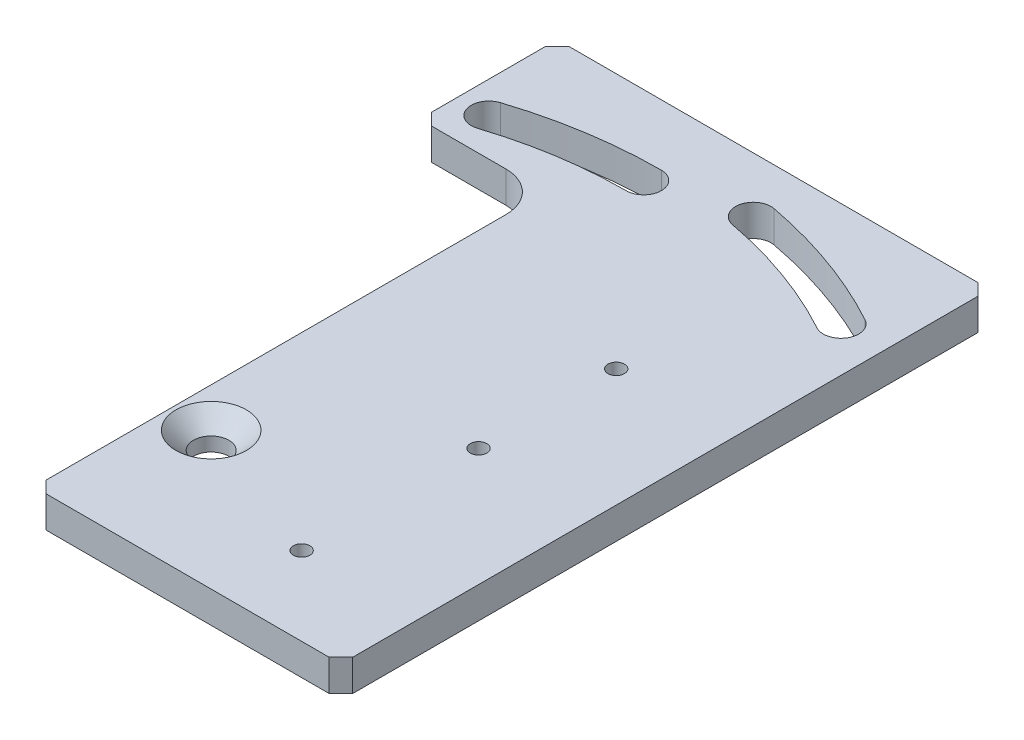
from build123d import *

# Parameters (mm, degrees)
SKETCH_1_W                   = 110
SKETCH_1_H                   = 165
EXTRUDE_1_DEPTH              = 8
SKETCH_2_W                   = 32
SKETCH_2_H                   = 130
CUT_EXTRUDE_1_DEPTH          = 8
HOLE_WIZARD_M8_1_D           = 9
HOLE_WIZARD_M8_1_DEPTH       = 10
HOLE_WIZARD_M8_1_CSINK_D     = 17.92
HOLE_WIZARD_M8_1_CSINK_ANGLE = 90
HOLE_WIZARD_M8_1_TIP         = 2.703872786
CUT_EXTRUDE_2_DEPTH          = 8
CUT_EXTRUDE_3_DEPTH          = 8
CHAMFER_1_SIZE               = 3
HOLE_WIZARD_M5_1_D           = 4.2
FILLET_1_R                   = 10


with BuildPart() as part:
    # 草图1 → 凸台-拉伸1 (new body)
    with BuildSketch(Plane(origin=(0, 0, 0), x_dir=(1, 0, 0), z_dir=(0, 1, 0))):
        Rectangle(SKETCH_1_W, SKETCH_1_H)
    extrude(amount=EXTRUDE_1_DEPTH)

    # 草图2 → 切除-拉伸1 (cut)
    with BuildSketch(Plane(origin=(0, 8, 0), x_dir=(1, 0, 0), z_dir=(0, 1, 0))):
        with Locations((-39, -17.5)):
            Rectangle(SKETCH_2_W, SKETCH_2_H)
    extrude(amount=-CUT_EXTRUDE_1_DEPTH, mode=Mode.SUBTRACT)

    # M8 六角凹锥坑螺钉的锥形沉头孔1
    with Locations(Plane(origin=(0, 8, 0), x_dir=(1, 0, 0), z_dir=(0, 1, 0))):
        with Locations((-13, -47.5)):
            CounterSinkHole(HOLE_WIZARD_M8_1_D / 2, HOLE_WIZARD_M8_1_CSINK_D / 2, depth=HOLE_WIZARD_M8_1_DEPTH, counter_sink_angle=HOLE_WIZARD_M8_1_CSINK_ANGLE)
            with Locations((0, 0, -(HOLE_WIZARD_M8_1_DEPTH + HOLE_WIZARD_M8_1_TIP / 2))):  # 118° drill point
                Cone(0, HOLE_WIZARD_M8_1_D / 2, HOLE_WIZARD_M8_1_TIP, mode=Mode.SUBTRACT)

    # 草图6 → 切除-拉伸2 (cut)
    with BuildSketch(Plane(origin=(0, 8, 0), x_dir=(1, 0, 0), z_dir=(0, 1, 0))):
        with BuildLine():
            ThreePointArc((-13, 67), (-30.911746247, 65.590314998), (-48.382445856, 61.395971116))
            ThreePointArc((-48.382445856, 61.395971116), (-51.271623705, 55.725640318), (-45.601292907, 52.836462469))
            ThreePointArc((-45.601292907, 52.836462469), (-29.503836062, 56.701119933), (-13, 58))
            ThreePointArc((-13, 58), (-8.5, 62.5), (-13, 67))
        make_face()
    extrude(amount=-CUT_EXTRUDE_2_DEPTH, mode=Mode.SUBTRACT)

    # 草图6<3> → 切除-拉伸3 (cut)
    with BuildSketch(Plane(origin=(0, 8, 0), x_dir=(1, 0, 0), z_dir=(0, 1, 0))):
        with BuildLine():
            ThreePointArc((-13, 67), (-30.911746247, 65.590314998), (-48.382445856, 61.395971116))
            ThreePointArc((-48.382445856, 61.395971116), (-51.271623705, 55.725640318), (-45.601292907, 52.836462469))
            ThreePointArc((-45.601292907, 52.836462469), (-29.503836062, 56.701119933), (-13, 58))
            ThreePointArc((-13, 58), (-8.5, 62.5), (-13, 67))
        make_face()
        with BuildLine():
            ThreePointArc((45.83353556, 59.947033898), (28.30077784, 67.827775275), (9.751057901, 72.868764073))
            ThreePointArc((9.751057901, 72.868764073), (4.493595053, 69.282807519), (8.079551606, 64.025344671))
            ThreePointArc((8.079551606, 64.025344671), (25.266434979, 59.354714234), (41.511071723, 52.052966102))
            ThreePointArc((41.511071723, 52.052966102), (47.61933754, 53.838768081), (45.83353556, 59.947033898))
        make_face()
    extrude(amount=-CUT_EXTRUDE_3_DEPTH, mode=Mode.SUBTRACT)

    # 倒角1
    chamfer_1_edges = [part.edges().sort_by_distance(p)[0] for p in [
        (-55, 4, -47.5),
        (-23, 4, 82.5),
        (55, 4, 82.5),
        (-55, 4, -82.5),
        (55, 4, -82.5),
    ]]
    chamfer(chamfer_1_edges, length=CHAMFER_1_SIZE)

    # M5 螺纹孔1 (through all)
    with Locations(Plane(origin=(0, 8, 0), x_dir=(1, 0, 0), z_dir=(0, 1, 0))):
        with Locations((25, -62.5), (25, -17.5), (25, 17.5)):
            Hole(HOLE_WIZARD_M5_1_D / 2)

    # 圆角1
    fillet_1_edges = [part.edges().sort_by_distance(p)[0] for p in [
        (-23, 4, -47.5),
    ]]
    fillet(fillet_1_edges, radius=FILLET_1_R)


solid = part.part
